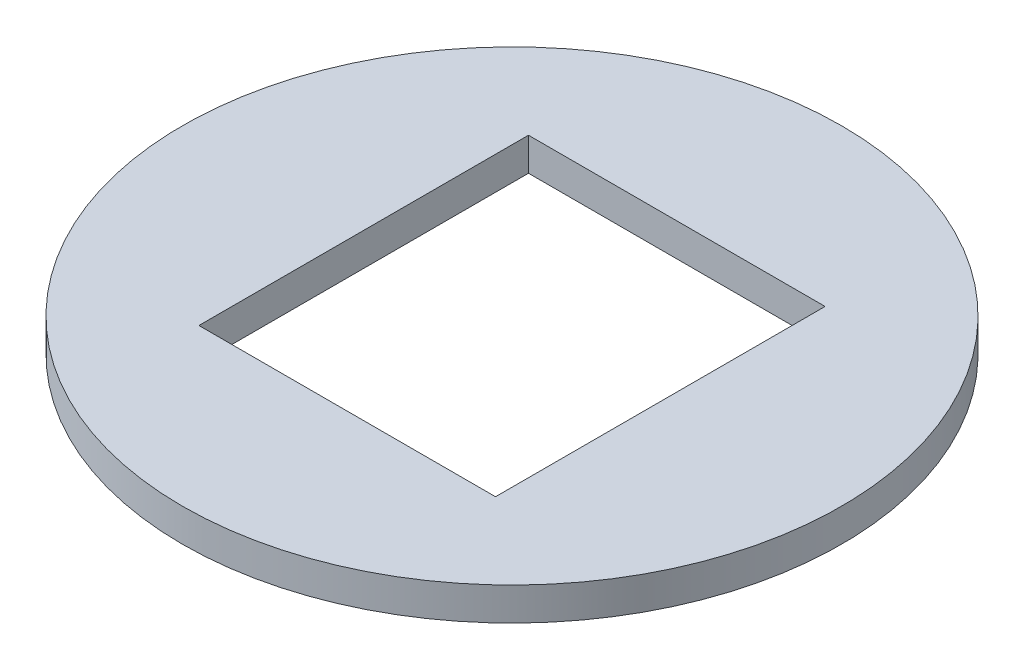
from build123d import *

# Parameters (mm, degrees)
SKETCH1_R               = 500
BOSS_EXTRUDE1_DEPTH     = 50
CUT_EXTRUDE1_DEPTH      = 709.872343938
CUT_EXTRUDE1_DEPTH_BACK = 709.872343938
SKETCH2_W               = 450
SKETCH2_H               = 500


with BuildPart() as part:
    # Sketch1 → Boss-Extrude1 (new body)
    with BuildSketch(Plane(origin=(0, 0, 0), x_dir=(1, 0, 0), z_dir=(0, 1, 0))):
        with Locations(Location((0, 0, 0), (0, 0, 270))):
            Circle(SKETCH1_R)
    extrude(amount=BOSS_EXTRUDE1_DEPTH)

    # Sketch2 → Cut-Extrude1 (cut, two sides: drawn at the far end of the back side and taken through both)
    with BuildSketch(Plane(origin=(0, 50, 0), x_dir=(1, 0, 0), z_dir=(0, 1, 0)).offset(-CUT_EXTRUDE1_DEPTH_BACK)):
        Rectangle(SKETCH2_W, SKETCH2_H)
    extrude(amount=CUT_EXTRUDE1_DEPTH + CUT_EXTRUDE1_DEPTH_BACK, mode=Mode.SUBTRACT)


solid = part.part
